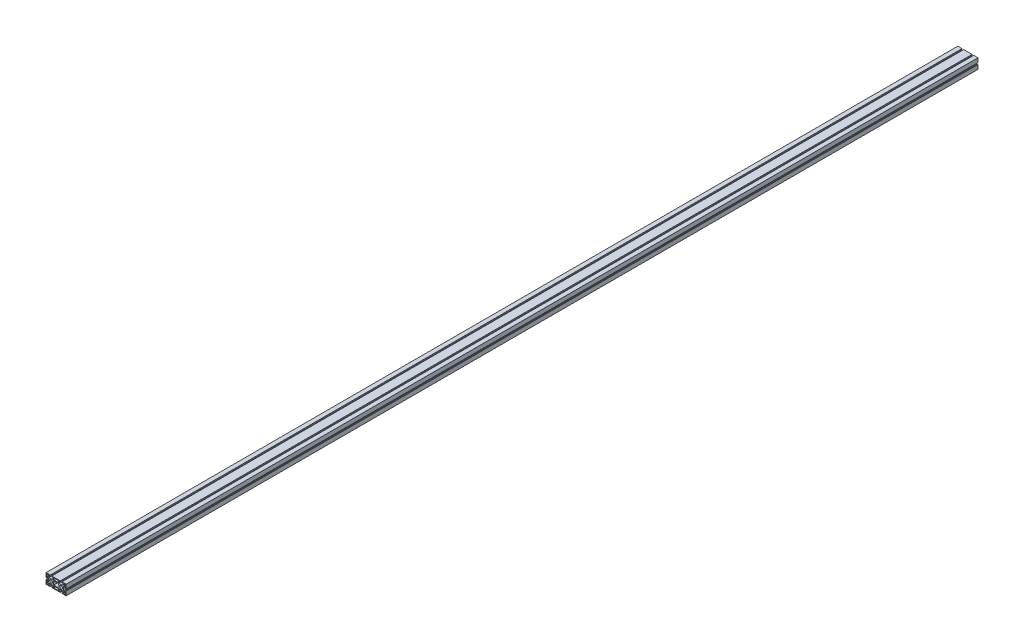
from build123d import *

# Parameters (mm, degrees)
SKETCH_1_R          = 4.1077368
SKETCH_1_W          = 5
SKETCH_1_H          = 5
EXTRUDE_1_DEPTH     = 2720
SKETCH_2_W          = 4
SKETCH_2_H          = 5
CUT_EXTRUDE_1_DEPTH = 2721.827080136
SKETCH_3_W          = 4
SKETCH_3_H          = 11
CUT_EXTRUDE_2_DEPTH = 2721.827080136


with BuildPart() as part:
    # 草图1 → 拉伸1 (new body)
    with BuildSketch(Plane.XY):
        with BuildLine():
            Line((12.5, 0), (12.5, -2))
            Line((12.5, -2), (9.5, -2))
            Line((9.5, -2), (9.5, -7))
            ThreePointArc((9.5, -7), (15, -8.308258509), (20.5, -7))
            Line((20.5, -7), (20.5, -2))
            Line((20.5, -2), (17.5, -2))
            Line((17.5, -2), (17.5, 0))
            Line((17.5, 0), (42.5, 0))
            Line((42.5, 0), (42.5, -2))
            Line((42.5, -2), (39.5, -2))
            Line((39.5, -2), (39.5, -7))
            ThreePointArc((39.5, -7), (45, -8.308258509), (50.5, -7))
            Line((50.5, -7), (50.5, -2))
            Line((50.5, -2), (47.5, -2))
            Line((47.5, -2), (47.5, 0))
            Line((47.5, 0), (60, 0))
            Line((60, 0), (60, -12.5))
            Line((60, -12.5), (58, -12.5))
            Line((58, -12.5), (58, -9.5))
            Line((58, -9.5), (53, -9.5))
            ThreePointArc((53, -9.5), (51.691741491, -15), (53, -20.5))
            Line((53, -20.5), (58, -20.5))
            Line((58, -20.5), (58, -17.5))
            Line((58, -17.5), (60, -17.5))
            Line((60, -17.5), (60, -30))
            Line((60, -30), (47.5, -30))
            Line((47.5, -30), (47.5, -28))
            Line((47.5, -28), (50.5, -28))
            Line((50.5, -28), (50.5, -23))
            ThreePointArc((50.5, -23), (45, -21.691741491), (39.5, -23))
            Line((39.5, -23), (39.5, -28))
            Line((39.5, -28), (42.5, -28))
            Line((42.5, -28), (42.5, -30))
            Line((42.5, -30), (17.5, -30))
            Line((17.5, -30), (17.5, -28))
            Line((17.5, -28), (20.5, -28))
            Line((20.5, -28), (20.5, -23))
            ThreePointArc((20.5, -23), (15, -21.691741491), (9.5, -23))
            Line((9.5, -23), (9.5, -28))
            Line((9.5, -28), (12.5, -28))
            Line((12.5, -28), (12.5, -30))
            Line((12.5, -30), (0, -30))
            Line((0, -30), (0, -17.5))
            Line((0, -17.5), (2, -17.5))
            Line((2, -17.5), (2, -20.5))
            Line((2, -20.5), (7, -20.5))
            ThreePointArc((7, -20.5), (8.308258509, -15), (7, -9.5))
            Line((7, -9.5), (2, -9.5))
            Line((2, -9.5), (2, -12.5))
            Line((2, -12.5), (0, -12.5))
            Line((0, -12.5), (0, 0))
            Line((0, 0), (12.5, 0))
        make_face()
        with Locations((15, -15)):
            Circle(SKETCH_1_R, mode=Mode.SUBTRACT)
        with Locations(Location((45, -15, 0), (0, 0, 180))):
            Circle(SKETCH_1_R, mode=Mode.SUBTRACT)
        with BuildLine():
            Line((32, -12.5), (28, -12.5))
            Line((28, -12.5), (28, -9.5))
            Line((28, -9.5), (23, -9.5))
            ThreePointArc((23, -9.5), (21.691741491, -15), (23, -20.5))
            Line((23, -20.5), (28, -20.5))
            Line((28, -20.5), (28, -17.5))
            Line((28, -17.5), (32, -17.5))
            Line((32, -17.5), (32, -20.5))
            Line((32, -20.5), (37, -20.5))
            ThreePointArc((37, -20.5), (38.308258509, -15), (37, -9.5))
            Line((37, -9.5), (32, -9.5))
            Line((32, -9.5), (32, -12.5))
        make_face(mode=Mode.SUBTRACT)
        with Locations((55.5, -4.5)):
            Rectangle(SKETCH_1_W, SKETCH_1_H, mode=Mode.SUBTRACT)
        with Locations((25.5, -25.5)):
            Rectangle(SKETCH_1_W, SKETCH_1_H, mode=Mode.SUBTRACT)
        with Locations((25.5, -4.5)):
            Rectangle(SKETCH_1_W, SKETCH_1_H, mode=Mode.SUBTRACT)
        with Locations((4.5, -25.5)):
            Rectangle(SKETCH_1_W, SKETCH_1_H, mode=Mode.SUBTRACT)
        with Locations((4.5, -4.5)):
            Rectangle(SKETCH_1_W, SKETCH_1_H, mode=Mode.SUBTRACT)
        with Locations((55.5, -25.5)):
            Rectangle(SKETCH_1_W, SKETCH_1_H, mode=Mode.SUBTRACT)
        with Locations((34.5, -25.5)):
            Rectangle(SKETCH_1_W, SKETCH_1_H, mode=Mode.SUBTRACT)
        with Locations((34.5, -4.5)):
            Rectangle(SKETCH_1_W, SKETCH_1_H, mode=Mode.SUBTRACT)
    extrude(amount=EXTRUDE_1_DEPTH)

    # 草图2 → 切除-拉伸1 (cut, through all)
    with BuildSketch(Plane.XY.offset(2720)):
        with Locations((30, -4.5)):
            Rectangle(SKETCH_2_W, SKETCH_2_H)
        with Locations((30, -25.5)):
            Rectangle(SKETCH_2_W, SKETCH_2_H)
    extrude(amount=-CUT_EXTRUDE_1_DEPTH, mode=Mode.SUBTRACT)

    # 草图3 → 切除-拉伸2 (cut, through all)
    with BuildSketch(Plane.XY.offset(2720)):
        with Locations((30, -15)):
            Rectangle(SKETCH_3_W, SKETCH_3_H)
    extrude(amount=-CUT_EXTRUDE_2_DEPTH, mode=Mode.SUBTRACT)


solid = part.part
